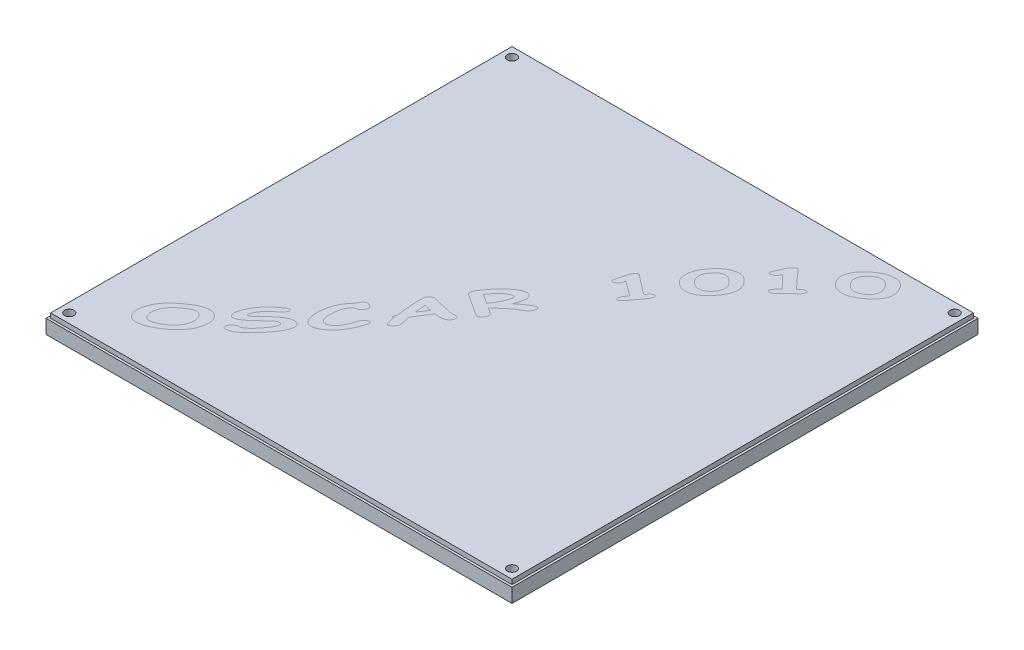
from build123d import *

# Parameters (mm, degrees)
SKETCH1_W           = 200
SKETCH1_H           = 200
SKETCH1_R           = 2
BOSS_EXTRUDE1_DEPTH = 6
SKETCH2_W           = 198
SKETCH2_H           = 198
BOSS_EXTRUDE2_DEPTH = 2
SKETCH4_R           = 2
CUT_EXTRUDE1_DEPTH  = 142.647449677


with BuildPart() as part:
    # Sketch1 → Boss-Extrude1 (new body)
    with BuildSketch(Plane(origin=(0, 0, 0), x_dir=(1, 0, 0), z_dir=(0, 1, 0))):
        Rectangle(SKETCH1_W, SKETCH1_H)
        with Locations(Location((95, 95, 0), (0, 0, 270))):
            Circle(SKETCH1_R, mode=Mode.SUBTRACT)
        with Locations(Location((95, -95, 0), (0, 0, 270))):
            Circle(SKETCH1_R, mode=Mode.SUBTRACT)
        with Locations(Location((-95, -95, 0), (0, 0, 270))):
            Circle(SKETCH1_R, mode=Mode.SUBTRACT)
        with Locations(Location((-95, 95, 0), (0, 0, 270))):
            Circle(SKETCH1_R, mode=Mode.SUBTRACT)
    extrude(amount=BOSS_EXTRUDE1_DEPTH)

    # Sketch2 → Boss-Extrude2 (add)
    with BuildSketch(Plane(origin=(0, 6, 0), x_dir=(1, 0, 0), z_dir=(0, 1, 0))):
        Rectangle(SKETCH2_W, SKETCH2_H)
    extrude(amount=BOSS_EXTRUDE2_DEPTH)

    # Sketch4 → Cut-Extrude1 (cut, through all)
    with BuildSketch(Plane(origin=(0, 8, 0), x_dir=(1, 0, 0), z_dir=(0, 1, 0))):
        with Locations(Location((-95, -95, 0), (0, 0, 270))):
            Circle(SKETCH4_R)
        with Locations(Location((95, -95, 0), (0, 0, 270))):
            Circle(SKETCH4_R)
        with Locations(Location((95, 95, 0), (0, 0, 270))):
            Circle(SKETCH4_R)
        with Locations(Location((-95, 95, 0), (0, 0, 270))):
            Circle(SKETCH4_R)
    extrude(amount=-CUT_EXTRUDE1_DEPTH, mode=Mode.SUBTRACT)


solid = part.part
